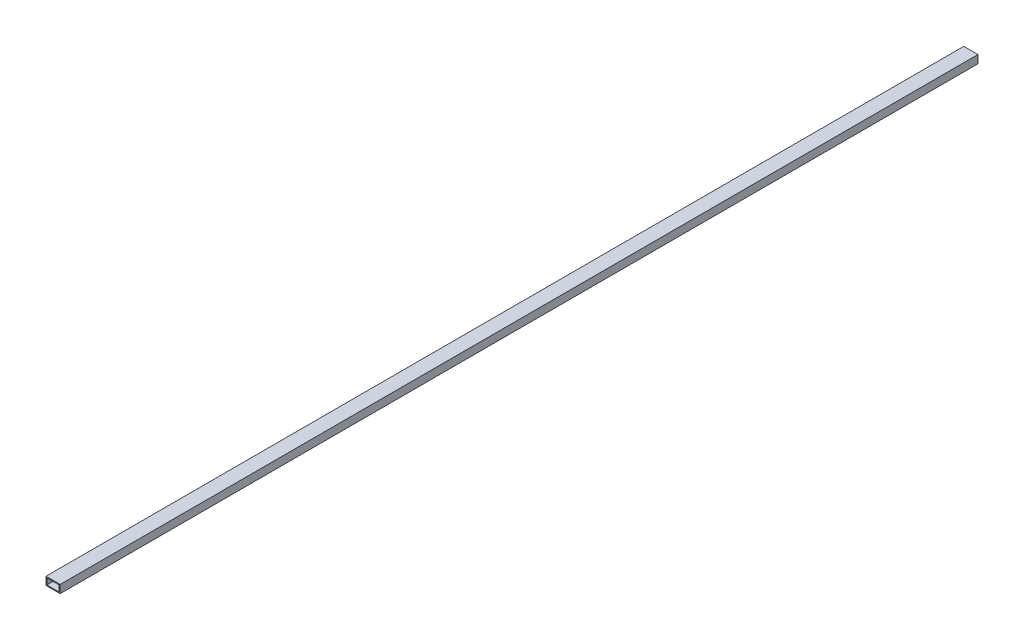
from build123d import *

# Parameters (mm, degrees)
SKETCH1_W           = 23
SKETCH1_H           = 13
SKETCH1_W_2         = 20
SKETCH1_H_2         = 10
EXTRUDE_THIN1_DEPTH = 1490


with BuildPart() as part:
    # Sketch1 → Extrude-Thin1 (new body)
    with BuildSketch(Plane.XY):
        with Locations((10, -5)):
            Rectangle(SKETCH1_W, SKETCH1_H)
        with Locations((10, -5)):
            Rectangle(SKETCH1_W_2, SKETCH1_H_2, mode=Mode.SUBTRACT)
    extrude(amount=EXTRUDE_THIN1_DEPTH)


solid = part.part
